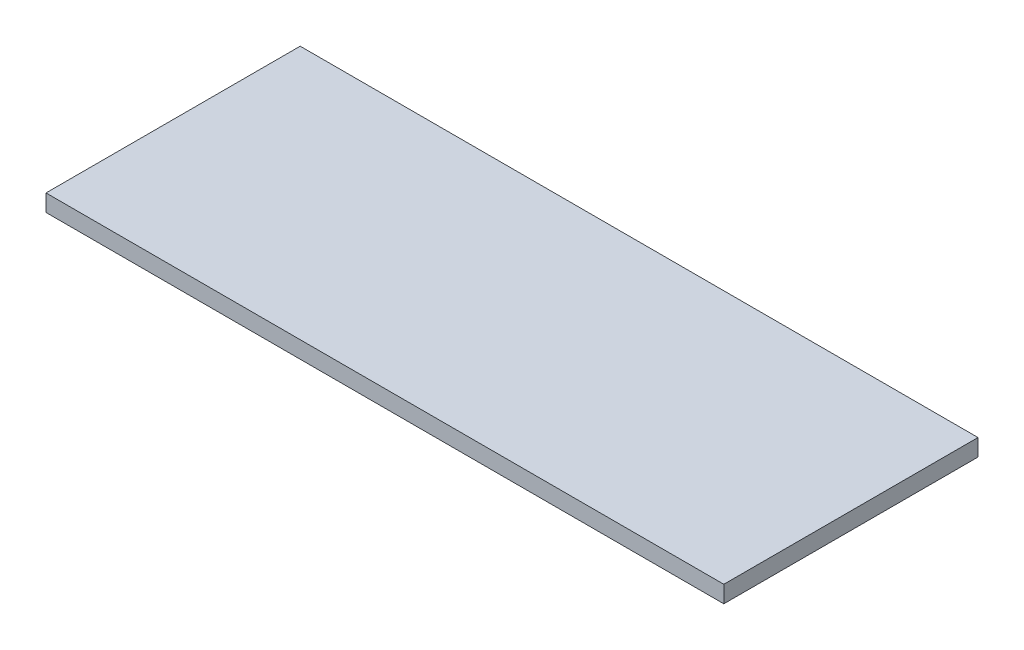
from build123d import *

# Parameters (mm, degrees)
SKETCH_1_W      = 40
SKETCH_1_H      = 15
EXTRUDE_1_DEPTH = 1


with BuildPart() as part:
    # 草图1 → 凸台-拉伸1 (new body)
    with BuildSketch(Plane(origin=(0, 0, 0), x_dir=(1, 0, 0), z_dir=(0, 1, 0))):
        Rectangle(SKETCH_1_W, SKETCH_1_H)
    extrude(amount=EXTRUDE_1_DEPTH)


solid = part.part
